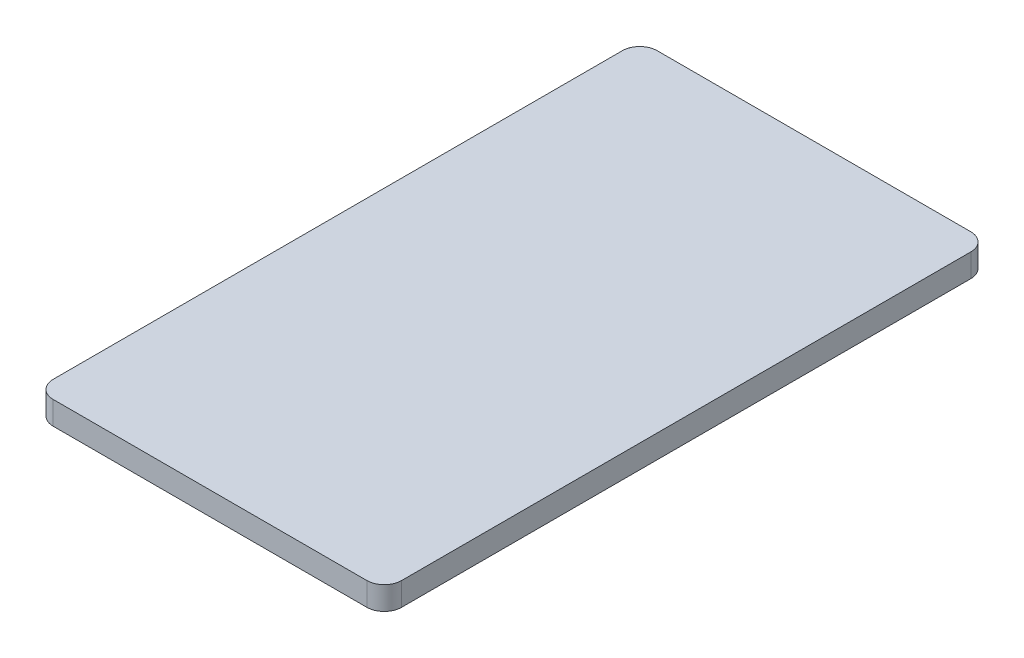
from build123d import *

# Parameters (mm, degrees)
BOSS_EXTRUDE_1_DEPTH = 20


with BuildPart() as part:
    # Sketch 1 → Boss-Extrude 1 (new body)
    with BuildSketch(Plane(origin=(0, 0, 0), x_dir=(1, 0, 0), z_dir=(0, 1, 0))):
        with BuildLine():
            Line((135, 260), (-135, 260))
            ThreePointArc((-135, 260), (-145.606601718, 255.606601718), (-150, 245))
            Line((-150, 245), (-150, -245))
            ThreePointArc((-150, -245), (-145.606601718, -255.606601718), (-135, -260))
            Line((-135, -260), (135, -260))
            ThreePointArc((135, -260), (145.606601718, -255.606601718), (150, -245))
            Line((150, -245), (150, 245))
            ThreePointArc((150, 245), (145.606601718, 255.606601718), (135, 260))
        make_face()
    extrude(amount=BOSS_EXTRUDE_1_DEPTH)


solid = part.part
